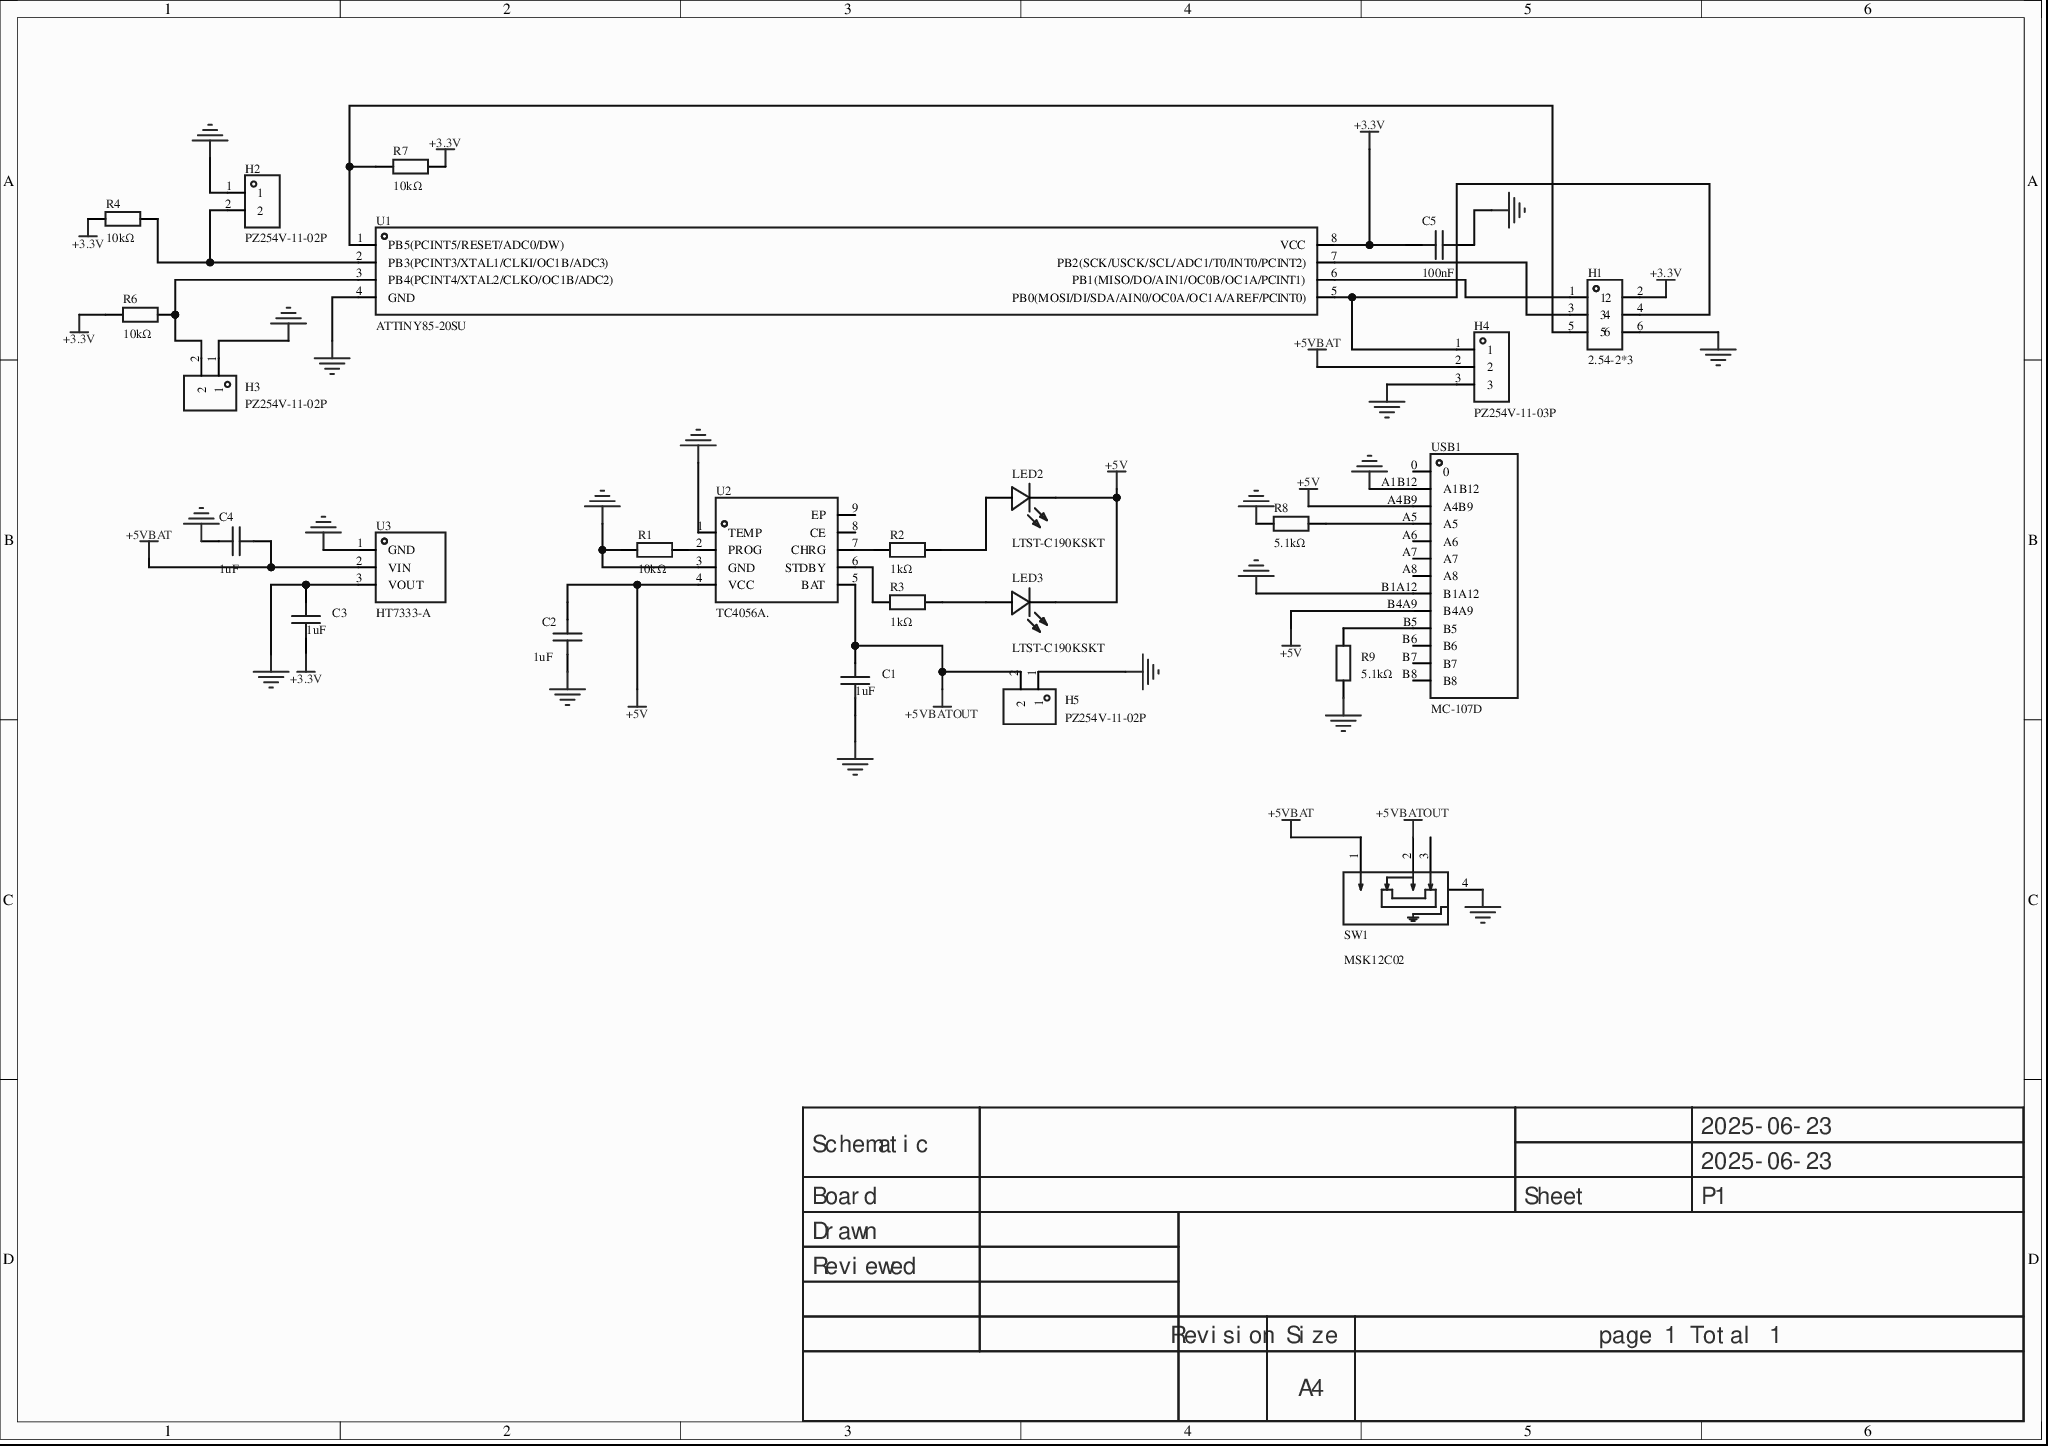
[diagram p0: MISC89049-3.schdoc]
# Altium project MISC89049-2.PrjPcb
1 sheet, 25 parts. Net scope: global (net labels, ports and power ports of the same name join across sheets).
Board file: MISC89049.pcbdoc

## Sheet MISC89049-3.schdoc
size 297 x 209 mm; Version: V1.0; @Project Name: MISC89049; @Page Count: 1; @Update Date: 2025-06-23; @Create Date: 2025-06-23; @Schematic Name: MISC89049; @Page No: 1; @Create Time: 01:15:29; @Update Time: 10:15:08; @Board Name: MISC89049

### Parts
C1  1uF  [C0603]
C2  1uF  [C0603]
C3  1uF  [C0603]
C4  1uF  [C0603]
C5  100nF  [C0603]
H1  2.54-2*3  [HDR-TH_6P-P2.54-V-R2-C3-S2.54_A2541WV-2X3P]
H2  PZ254V-11-02P  [HDR-TH_2P-P2.54-V-M]
H3  PZ254V-11-02P  [HDR-TH_2P-P2.54-V-M]
H4  PZ254V-11-03P  [HDR-TH_3P-P2.54-V-M]
H5  PZ254V-11-02P  [HDR-TH_2P-P2.54-V-M]
LED2  LTST-C190KSKT  [LED0603-RD]
LED3  LTST-C190KSKT  [LED0603-RD]
R1  10kΩ  [R0603]
R2  1kΩ  [R0603]
R3  1kΩ  [R0603]
R4  10kΩ  [R0603]
R6  10kΩ  [R0603]
R7  10kΩ  [R0603]
R8  5.1kΩ  [R0603]
R9  5.1kΩ  [R0603]
SW1  MSK12C02  [SW-TH_MSK12C02]
U1  ATTINY85-20SU  [SOIC-8_L5.3-W5.3-P1.27-LS8.0-BL]
U2  TC4056A.  [ESOP-8_L4.9-W3.9-P1.27-LS6.0-BL-EP]
U3  HT7333-A  [SOT-89-3_L4.5-W2.5-P1.50-LS4.2-BR]
USB1  MC-107D  [USB-C-SMD_MC-107D]

### Nets
+3.3V: C3.1 C5.2 H1.2 R4.2 R6.1 R7.2 U1.8(VCC)
+5V: C2.2 LED2.1(-) LED3.1(-) U2.4(VCC) USB1.A4B9 USB1.B4A9
+5VBAT: C4.1 H4.2 SW1.1 U3.2(VIN)
+5VBATOUT: C1.2 H5.2 SW1.2 U2.5(BAT)
GND: C1.1 C2.1 C3.2 C4.2 C5.1 H1.6 H2.1 H3.1 H4.3 H5.1 R1.1 R8.1 R9.2 SW1.4 U1.4(GND) U2.1(TEMP) U2.3(GND) U3.1(GND) U3.3(VOUT) USB1.A1B12 USB1.B1A12
NetH1_1: H1.1 U1.6(PB1(MISO/DO/AIN1/OC0B/OC1A/PCINT1))
NetH1_3: H1.3 U1.7(PB2(SCK/USCK/SCL/ADC1/T0/INT0/PCINT2))
NetH1_4: H1.4 H4.1 U1.5(PB0(MOSI/DI/SDA/AIN0/OC0A/OC1A/AREF/PCINT0))
NetH1_5: H1.5 R7.1 U1.1(PB5(PCINT5/RESET/ADC0/DW))
NetH2_2: H2.2 R4.1 U1.2(PB3(PCINT3/XTAL1/CLKI/OC1B/ADC3))
NetH3_2: H3.2 R6.2 U1.3(PB4(PCINT4/XTAL2/CLKO/OC1B/ADC2))
NetLED2_2: LED2.2(+) R2.2
NetLED3_2: LED3.2(+) R3.2
NetR1_2: R1.2 U2.2(PROG)
NetR2_1: R2.1 U2.7(CHRG)
NetR3_1: R3.1 U2.6(STDBY)
NetR8_2: R8.2 USB1.A5
NetR9_1: R9.1 USB1.B5

Not connected (* = marked no-connect by the designer): SW1 3; U2 8(CE) 9(EP); USB1 0 A6 A7 A8 B6 B7 B8

### Notes on the sheet
- 2025-06-23
- Schematic
- Board
- Sheet
- P1
- Drawn
- Reviewed
- Revision
- Size
- A4
- page 1 Total 1

### Library data of the parts
C1-C5 = CGA0603X5R105K500JT: Capacitance: 1uF; tolerance: ±10%; rated voltage: 50V; temperature coefficient: X5R;; Manufacturer: HRE(芯声); AddInBom: yes; ModelId: ac125912035d415993ca9572d50418b1; ModelName: C0603_L1.6-W0.8-H0.8; ModelTransform: 62.992,31.496,0,0,0,0,0,0,0; Symbol: CGA0603X5R105K500JT; Device: CGA0603X5R105K500JT; LCSC Part Name: 1uF ±10% 50V; ManufacturerPart: CGA0603X5R105K500JT; Supplier Footprint: 0603; JLCPCB Part Class: Extended library; Supplier: LCSC; ConvertToPcb: yes; FootprintName: C0603; Tolerance: ±10%; Voltage Rating: 50V; Temperature Coefficient: X5R
  C1-C4: SupplierPart: C6119852; Value: 1uF
  C5: Value: 100nF
H1 = 2.54-2*3: Pin structure: 2x3P; pitch: 2.54mm; rows: double row; total pins: 6P;; Manufacturer: ZHOURI(洲日); AddInBom: yes; ModelId: fd1b55b786fb415ca65c4187088147b7; ModelName: HDR2.54-M-LI-2x3P; ModelTransform: 299.9994,200,0,0,0,0,0,0,-118.11; Symbol: 2.54-2*3; Device: 2.54-2*3; LCSC Part Name: 2.54-2*3; SupplierPart: C5116479; ManufacturerPart: 2.54-2*3; Supplier Footprint: 插件,P=2.54mm; JLCPCB Part Class: Extended library; Datasheet: example.com/upload/public/pdf/source/20220729/7A96040568D3A9F25ED0F1D4F891C529.pdf; Supplier: LCSC; ConvertToPcb: yes; FootprintName: HDR-TH_6P-P2.54-V-R2-C3-S2.54_A2541WV-2X3P; Pin Structure: 2x3P; Pitch: 2.54mm; Number of Rows: Double row; Number of Pins: 6P
H2 H3 H5 = PZ254V-11-02P: Pin structure: 1x2P; pitch: 2.54mm; row spacing: -; round/square pin: square pin; mounting: through-hole; rows: single row; total pins: 2P; rated current: -; rated voltage: -; mating pin length: 6mm; plastic height: 2.5mm; tail length: 3mm; contact material: brass; contact plating: -; operating temperature: -40℃~+105℃; color: black;; Manufacturer: XFCN(兴飞); AddInBom: yes; ModelId: e35305ec3aa84b66b849f914b715e73f; ModelName: HDR2.54-M-LI-1X2P; ModelTransform: 200,100,0,0,0,0,0,0,-118.11; Symbol: PZ254V-11-02P; Device: PZ254V-11-02P; LCSC Part Name: 1x2P 间距:2.54mm 方针 直插; SupplierPart: C492401; ManufacturerPart: PZ254V-11-02P; Supplier Footprint: 插件,P=2.54mm; JLCPCB Part Class: Extended library; Datasheet: example.com/upload/public/pdf/source/20200309/C492401_A812433581A9B211A7FFA413ADDFF0E5.pdf; Supplier: LCSC; ConvertToPcb: yes; FootprintName: HDR-TH_2P-P2.54-V-M; Pin Structure: 1x2P; Pitch: 2.54mm; Row Spacing: -; Circluar Pins/Square Pins: Square pin; Mounting Type: Through-hole; Number of Rows: Single row; Number of Pins: 2P; Current Rating: -; Voltage Rating (Max): -; Length of Mating Pin: 6mm; Insulation Height: 2.5mm; Length of End Connection Pin: 3mm; Contact Material: Brass; Contact Plating: -; Operating Temperature: -40℃~+105℃; Color: Black
H4 = PZ254V-11-03P: Pin structure: 1x3P; pitch: 2.54mm; row spacing: -; round/square pin: square pin; mounting: through-hole; rows: single row; total pins: 3P; rated current: 3A; rated voltage: 250V; mating pin length: 6mm; plastic height: 2.5mm; tail length: 3mm; operating temperature: -40℃~+105℃; color: black;; Manufacturer: XFCN(兴飞); Symbol: PZ254V-11-03P_C2937625; AddInBom: yes; ModelId: bb473b6d38ff42a99216a4fcdbdcc4cb; ModelName: HDR-TH_3P-P2.54-M-LI-1X3P; ModelTransform: 299.9994,100,0,0,0,0,0,0,-118.11; Device: PZ254V-11-03P; LCSC Part Name: 1x3P 间距:2.54mm 方针 直插; SupplierPart: C2937625; ManufacturerPart: PZ254V-11-03P; Supplier Footprint: 插件,P=2.54mm; JLCPCB Part Class: Extended library; Datasheet: example.com/upload/public/pdf/source/20200309/C492402_8335C3D49C4E4C618838D59BB1D024C1.pdf; Supplier: LCSC; ConvertToPcb: yes; FootprintName: HDR-TH_3P-P2.54-V-M; Pin Structure: 1x3P; Pitch: 2.54mm; Row Spacing: -; Circluar Pins/Square Pins: Square pin; Mounting Type: Through-hole; Number of Rows: Single row; Number of Pins: 3P; Current Rating: 3A; Voltage Rating (Max): 250V; Length of Mating Pin: 6mm; Insulation Height: 2.5mm; Length of End Connection Pin: 3mm; Operating Temperature: -40℃~+105℃; Color: Black
LED2 LED3 = LTST-C190KSKT: Emitted color: yellow; forward voltage (VF): 2.1V; power: 75mW; forward current: 20mA; dominant wavelength: 584.5nm~597nm; diode configuration: -; lens color: colorless transparent lens; color temperature: -; luminous intensity: 104mcd; viewing angle: 130°; tape and reel: -; operating temperature: -30℃~+85℃;; Manufacturer: LITEON(光宝); AddInBom: yes; ModelId: 1f0d29a91be547639d425604e9b96ebb; ModelTransform: 63.7794,32.283,0,0,0,0,0,0,0; Peak Wavelength: 588nm; Symbol: LTST-C190KSKT; Device: LTST-C190KSKT; LCSC Part Name: 黄灯; SupplierPart: C125095; ManufacturerPart: LTST-C190KSKT; Supplier Footprint: 0603; JLCPCB Part Class: Extended library; Datasheet: example.com/upload/public/pdf/source/20180129/C125095_15171881843821315881.pdf; Supplier: LCSC; ConvertToPcb: yes; FootprintName: LED0603-RD; ModelName: LED0603-RD; Emitted Color: Yellow; Forward Voltage (VF): 2.1V; Power Dissipation: 75mW; Forward Current: 20mA; Dominant Wavelength: 584.5nm~597nm; Diode Configuration: -; Lens Color: Colorless transparent lens; Color Temperature: -; Luminous Intensity: 104mcd; Viewing Angle: 130°; Mounting Sytle: -; Operating Temperature: -30℃~+85℃
R1-R4 R6-R9 = 0603WAF1002T5E: Resistor type: thick film resistor; resistance: 10kΩ; tolerance: ±1%; power: 100mW; working voltage: 75V; temperature coefficient: ±100ppm/℃;; Manufacturer: UNI-ROYAL(厚声); AddInBom: yes; ModelId: fc143cca1e79419f9cd78b61e9279f08; ModelTransform: 31.8897,63.7794,0,90,0,0,0,0,0; Symbol: 0603WAF1002T5E; Device: 0603WAF1002T5E; LCSC Part Name: 厚膜电阻 10kΩ ±1% 100mW; ManufacturerPart: 0603WAF1002T5E; Supplier Footprint: 0603; JLCPCB Part Class: Basic library; Datasheet: example.com/upload/public/pdf/source/20200306/C422600_1E6D84923E4A46A82E41ADD87F860B5C.pdf; Supplier: LCSC; ConvertToPcb: yes; FootprintName: R0603; ModelName: R0603; Type: Thick film resistor; Tolerance: ±1%; Power(Watts): 100mW; Voltage-Supply(Max): 75V; Temperature Coefficient: ±100ppm/℃; Operating Temperature: -55℃~+155℃
  R1: SupplierPart: C25804; Value: 10kΩ
  R2 R3: Value: 1kΩ
  R4 R6 R7: Value: 10kΩ
  R8 R9: Value: 5.1kΩ
SW1 = MSK12C02: Circuit structure: SPDT; mounting: lay-flat SMD; switch color: -; rated current (DC): 50mA; rated voltage (DC): 12V; rated current (AC): -; rated voltage (AC): -; mechanical life: 1万 cycles;; Manufacturer: SHOU HAN(首韩); AddInBom: yes; ModelId: fac986d38b354d44b3f0357550471109; ModelName: SW-SMD_3P-L6.6-W2.7-LS7.8-P1.50; ModelTransform: 307.086,204.724,0,180,0,0,0.001,-29.53,-19.685; Pin Style: SMD tab; Switch Length: 8mm; Switch Width: 2.8mm; Switch Height: 1.4mm; Symbol: MSK12C02; Device: MSK12C02; LCSC Part Name: 两档侧拨贴片 7脚 滑动开关; SupplierPart: C431540; ManufacturerPart: MSK12C02; Supplier Footprint: SMD; JLCPCB Part Class: Extended library; Datasheet: example.com/upload/public/pdf/source/20190925/C431540_89155AEF0758B9AD1B2D805F83FB12E3.pdf; Supplier: LCSC; ConvertToPcb: yes; FootprintName: SW-TH_MSK12C02; Circuit: SPDT; Actuator Style: -; Mounting Style: Lay-flat SMD; Actuator Color: -; Current Rating (DC): 50mA; Voltage Rating (DC): 12V; Current Rating (AC): -; Voltage Rating (AC): -; Mechanical Life: 1万 cycles; Operating Temperature: -20℃~+70℃
U1 = ATTINY85-20SU_C31540447: Manufacturer: MICROCHIP(美国微芯); AddInBom: yes; ModelId: f83d990ad74f400caf5ac920b7771508; ModelName: SOIC-8_L5.3-W5.3-H1.9-LS7.9-P1.27; ModelTransform: 208.661,311.25654,0,0,0,0,-0.0005,0.0005,0; Symbol: ATTINY85-20SU_C31540447; Device: ATTINY85-20SU_C31540447; LCSC Part Name: ATTINY85-20SU; SupplierPart: C31540447; ManufacturerPart: ATTINY85-20SU; Supplier Footprint: SOIC-8-208mil; JLCPCB Part Class: Extended library; Datasheet: example.com/upload/public/pdf/source/20220128/C2054451_C9B4ABB36EE91A4310FC2804A278EDC5.pdf; Supplier: LCSC; ConvertToPcb: yes; FootprintName: SOIC-8_L5.3-W5.3-P1.27-LS8.0-BL
U2 = TC4056A.: Manufacturer: FM(富满); AddInBom: yes; ModelId: d3e00daa36c445139c055a3b9efb85d2; ModelName: ESOP-8_L4.9-W3.9-H1.6-LS6.0-P1.27; ModelTransform: 240.157,192.913,0,90,0,0,0,0,0; Symbol: TC4056A.; Device: TC4056A.; LCSC Part Name: TC4056A.; SupplierPart: C7588528; ManufacturerPart: TC4056A.; Supplier Footprint: ESOP-8; JLCPCB Part Class: Extended library; Datasheet: example.com/upload/public/pdf/source/20230920/E3CE03BFF354F1B852E5B8FAF3A3EC05.pdf; Supplier: LCSC; ConvertToPcb: yes; FootprintName: ESOP-8_L4.9-W3.9-P1.27-LS6.0-BL-EP
U3 = HT7333-A_C347191: Output type: fixed; max input voltage: 12V; output voltage: 3.3V; output current: 250mA; power supply rejection ratio (PSRR): -; output polarity: positive;; Manufacturer: UMW(友台半导体); AddInBom: yes; ModelId: 6db690b7897d4d18a30d90c1b89525ee; ModelName: SOT-89-3_L4.3-W2.5-H1.6-LS4.1-P1.50; ModelTransform: 161.417,169.291,0,180,0,0,-11.808,0,0; Dropout Voltage: 90mV@(40mA); standby current: 3uA; Number of Outputs: 1; Symbol: HT7333-A_C347191; Device: HT7333-A_C347191; LCSC Part Name: 输入12V 输出3.3V 250mA; SupplierPart: C347191; ManufacturerPart: HT7333-A; Supplier Footprint: SOT-89-3; JLCPCB Part Class: Extended library; Datasheet: example.com/upload/public/pdf/source/20240108/E0D11255E13C966C6280704C6AF597A1.pdf; Supplier: LCSC; ConvertToPcb: yes; FootprintName: SOT-89-3_L4.5-W2.5-P1.50-LS4.2-BR; Output Type: Fixed; Maximum Input Voltage: 12V; Output Voltage: 3.3V; Output Current: 250mA; Power Supply Rejection Ratio (PSRR): -; Operating Temperature: -25℃~+70℃; Output Polarity: Positive
USB1 = MC-107D: Connector type: Type-C; standard: USB 3.1; gender: female; number of ports: 1; number of contacts: 16P; mounting: lay-flat SMD; rated current - power: 3A; contact material: -; contact plating: -; operating temperature range: -25℃~+85℃; soldering temperature (max): -;; Manufacturer: HANBO(汉博); AddInBom: yes; ModelId: 2fe00898b48b40e9be0875c04db047ee; ModelTransform: 351.9678,301.181,0,0,0,0,0,-40.157,-35.433; Number of Ports: 1; Symbol: MC-107D; Device: MC-107D; LCSC Part Name: Type-C 母 卧贴; SupplierPart: C2874568; ManufacturerPart: MC-107D; Supplier Footprint: SMD; JLCPCB Part Class: Extended library; Datasheet: example.com/upload/public/pdf/source/20221111/259210CA5C7DD1E901D76AB583C291FC.pdf; Supplier: LCSC; ConvertToPcb: yes; FootprintName: USB-C-SMD_MC-107D; ModelName: USB-C-SMD_MC-107D; Connector Type: Type-C; Standard: USB 3.1; Gender: Female; Number of Contacts: 16P; Mounting Style: Lay-flat SMD; Current Rating - Power (Max): 3A; Contact Material: -; Contact Plating: -; Operating Temperature Range: -25℃~+85℃; Soldering Temperature(Max): -